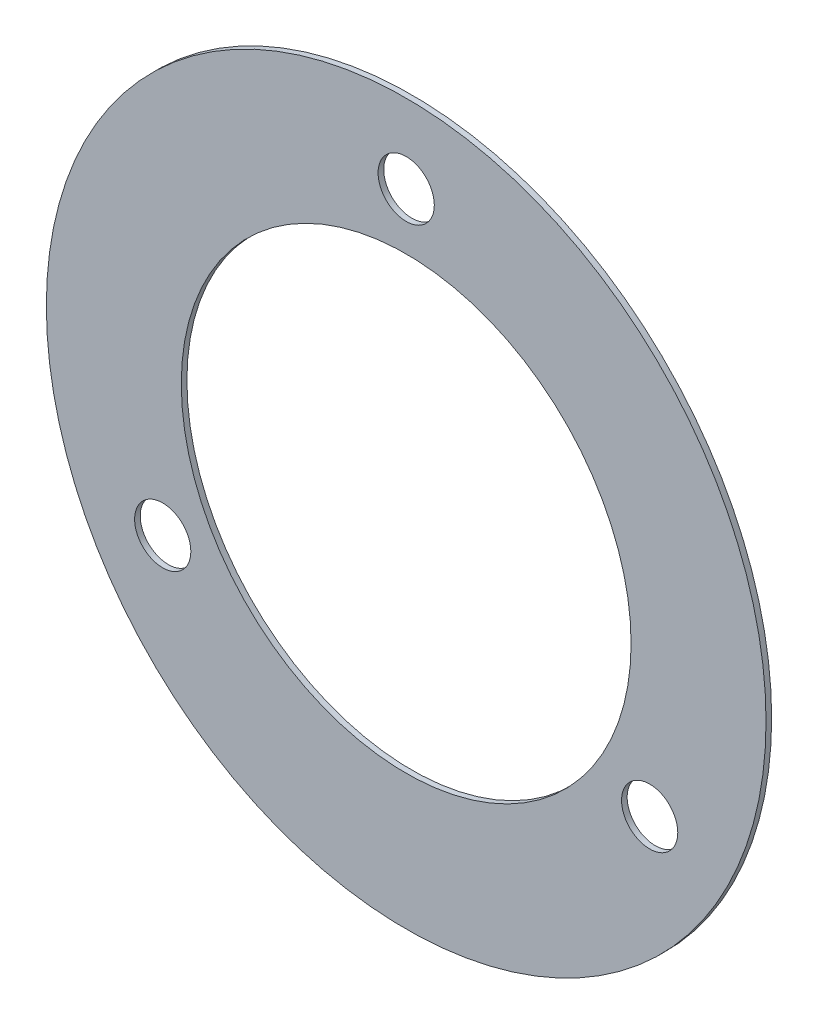
SolidWorks part; units mm, degrees
ref_plane "Front Plane" through (0, 0, 0) normal (0, 0, 1) x (1, 0, 0)
ref_plane "Top Plane" through (0, 0, 0) normal (0, 1, 0) x (1, 0, 0)
ref_plane "Right Plane" through (0, 0, 0) normal (1, 0, 0) x (0, 0, -1)
other "Configuration Table"
sketch "Sketch1" plane through (0, 0, 0) normal (0, 0, 1) x (1, 0, 0)
  circle A0 centre (0, 0) radius 32
  circle A1 centre (0, 0) radius 20
  dimension "D1" = 64
  dimension "D2" = 40
extrude "Boss-Extrude1" add sketch "Sketch1" along normal blind 0.5
sketch "Sketch2" plane through (0, 0, 0.5) normal (0, 0, 1) x (1, 0, 0)
  circle A0 centre (0, 0) radius 25 construction
  circle A1 centre (0, 25) radius 2.5
  circle A2 centre (21.6506, -12.5) radius 2.5
  circle A3 centre (-21.6506, -12.5) radius 2.5
  point P11 (0, 0)
  dimension "D1" = 50
  dimension "D2" = 5
  dimension "D3" = 3
extrude "Cut-Extrude1" cut sketch "Sketch2" against normal blind 0.5
